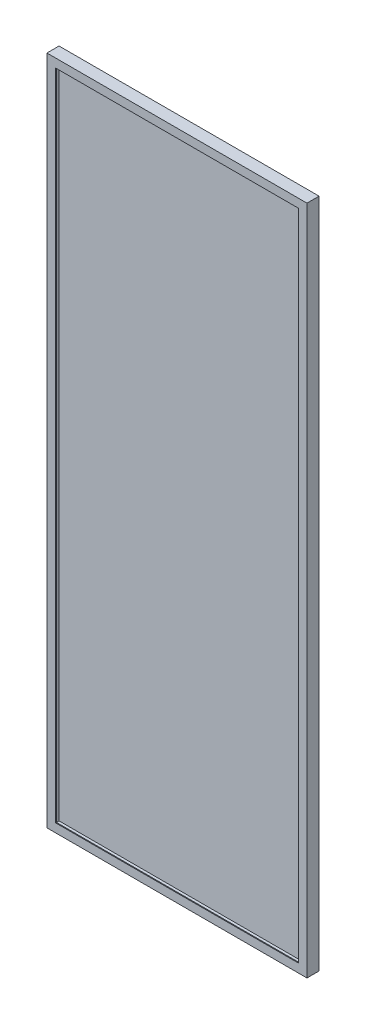
SolidWorks part; units mm, degrees
ref_plane "前视基准面" through (0, 0, 0) normal (0, 0, 1) x (1, 0, 0)
ref_plane "上视基准面" through (0, 0, 0) normal (0, 1, 0) x (1, 0, 0)
ref_plane "右视基准面" through (0, 0, 0) normal (1, 0, 0) x (0, 0, -1)
sketch "草图1" plane through (0, 0, 0) normal (0, 0, 1) x (1, 0, 0)
  line L1 (0, 0) -> (601, 0)
  line L2 (0, 0) -> (0, 1551)
  line L3 (0, 1551) -> (601, 1551)
  line L4 (601, 0) -> (601, 1551)
  dimension "D1" = 1551
  dimension "D2" = 601
extrude "凸台-拉伸1" add sketch "草图1" along normal blind 28
shell "抽壳1" thickness 2
sketch "草图2" plane through (0, 0, 28) normal (0, 0, 1) x (1, 0, 0)
  line L14 (20, 1531) -> (20, 20)
  line L15 (20, 20) -> (581, 20)
  line L16 (581, 20) -> (581, 1531)
  line L17 (581, 1531) -> (20, 1531)
  line L18 (20, 1531) -> (20, 20)
  line L19 (20, 20) -> (581, 20)
  line L20 (581, 20) -> (581, 1531)
  line L21 (581, 1531) -> (20, 1531)
  line L26 (0, 1551) -> (0, 0)
  line L27 (0, 0) -> (601, 0)
  line L28 (601, 0) -> (601, 1551)
  line L29 (601, 1551) -> (0, 1551)
  line L30 (0, 1551) -> (0, 0)
  line L31 (0, 0) -> (601, 0)
  line L32 (601, 0) -> (601, 1551)
  line L33 (601, 1551) -> (0, 1551)
  dimension "D1" = 20
  dimension "D2" = 0
extrude "凸台-拉伸2" add sketch "草图2" against normal blind 2
